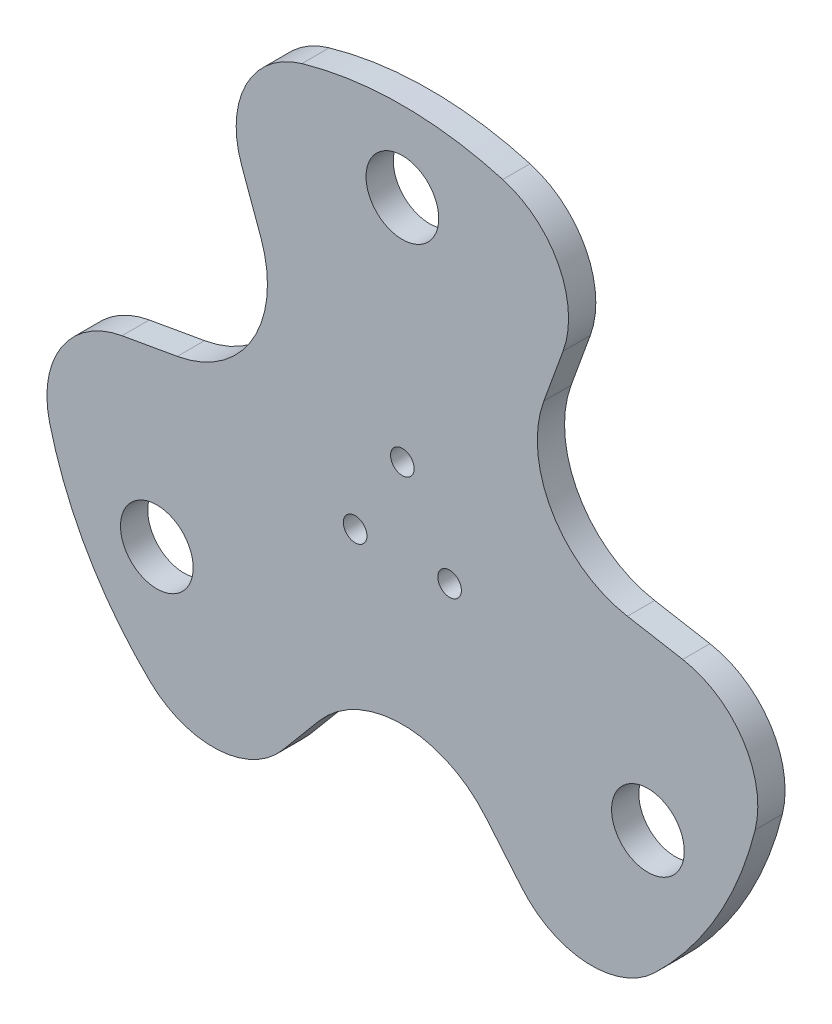
SolidWorks part; units mm, degrees
ref_plane "Front Plane" through (0, 0, 0) normal (0, 0, 1) x (1, 0, 0)
ref_plane "Top Plane" through (0, 0, 0) normal (0, 1, 0) x (1, 0, 0)
ref_plane "Right Plane" through (0, 0, 0) normal (1, 0, 0) x (0, 0, -1)
sketch "Sketch1" plane through (0, 0, 0) normal (0, 0, 1) x (1, 0, 0)
  circle A0 centre (0, 0) radius 200
  circle A1 centre (0, 156) radius 20
  circle A2 centre (135.1, -78) radius 20
  circle A3 centre (-135.1, -78) radius 20
  circle A5 centre (0, 30) radius 10.5 construction
  circle A6 centre (0, -30) radius 10.5 construction
  point P14 (0, 0)
  dimension "D1" = 400
  dimension "D3" = 40
  dimension "D6" = 21
  dimension "D2" = 156
  dimension "D5" = 60
  dimension "D7" = 30
  dimension "D4" = 3
extrude "Boss-Extrude1" add sketch "Sketch1" along normal blind 15
sketch "Sketch2" plane through (0, 0, 15) normal (0, 0, 1) x (1, 0, 0)
  line L0 (0, 0) -> (0, 155) construction
  line L1 (0, 0) -> (102.9043, 0) construction
  line L2 (-45.9627, 116.4327) -> (-177.6513, 273.3731) construction
  line L3 (-177.6513, 273.3731) -> (100.686, 181.6495) construction
  line L4 (100.686, 181.6495) -> (45.9627, 116.4327) construction
  line L14 (-45.9627, -116.4327) -> (-177.6513, -273.3731)
  line L15 (-177.6513, -273.3731) -> (100.686, -181.6495)
  line L16 (100.686, -181.6495) -> (45.9627, -116.4327)
  line L17 (-77.8524, 98.0212) -> (-147.9224, 290.5371)
  line L18 (-147.9224, 290.5371) -> (-207.6561, 3.6281)
  line L19 (-207.6561, 3.6281) -> (-123.815, 18.4115)
  line L20 (123.815, 18.4115) -> (325.5737, -17.164)
  line L21 (325.5737, -17.164) -> (106.9701, 178.0214)
  line L22 (106.9701, 178.0214) -> (77.8524, 98.0212)
  arc A0 (-45.9627, 116.4327) -> (45.9627, 116.4327) centre (0, 155) ccw construction
  arc A4 (-45.9627, -116.4327) -> (45.9627, -116.4327) centre (0, -155) cw
  arc A5 (-77.8524, 98.0212) -> (-123.815, 18.4115) centre (-134.2339, 77.5) cw
  arc A6 (123.815, 18.4115) -> (77.8524, 98.0212) centre (134.2339, 77.5) cw
  point P25 (0, 0)
  point P26 (0, 0)
  dimension "D3" = 120
  dimension "D1" = 90
  dimension "D2" = 155
  dimension "D4" = 40
  dimension "D6" = 293.0612
  dimension "D7" = 156.9404
  dimension "D5" = 3
extrude "Cut-Extrude1" cut sketch "Sketch2" against normal blind 30
fillet "Fillet1" radius 50 6 edges at (-95.6482, -175.6457, 7.5) (95.6482, -175.6457, 7.5) (199.9378, 4.989, 7.5) (104.2895, 170.6567, 7.5) (-199.9378, 4.989, 7.5) (-104.2895, 170.6567, 7.5)
sketch "Sketch3" plane through (0, 0, 15) normal (0, 0, 1) x (1, 0, 0)
  circle A0 centre (0, 30) radius 6.5
  circle A1 centre (25.9808, -15) radius 6.5
  circle A2 centre (-25.9808, -15) radius 6.5
  point P9 (0, 0)
  dimension "D1" = 13
  dimension "D2" = 30
  dimension "D3" = 3
extrude "Cut-Extrude2" cut sketch "Sketch3" against normal blind 50
